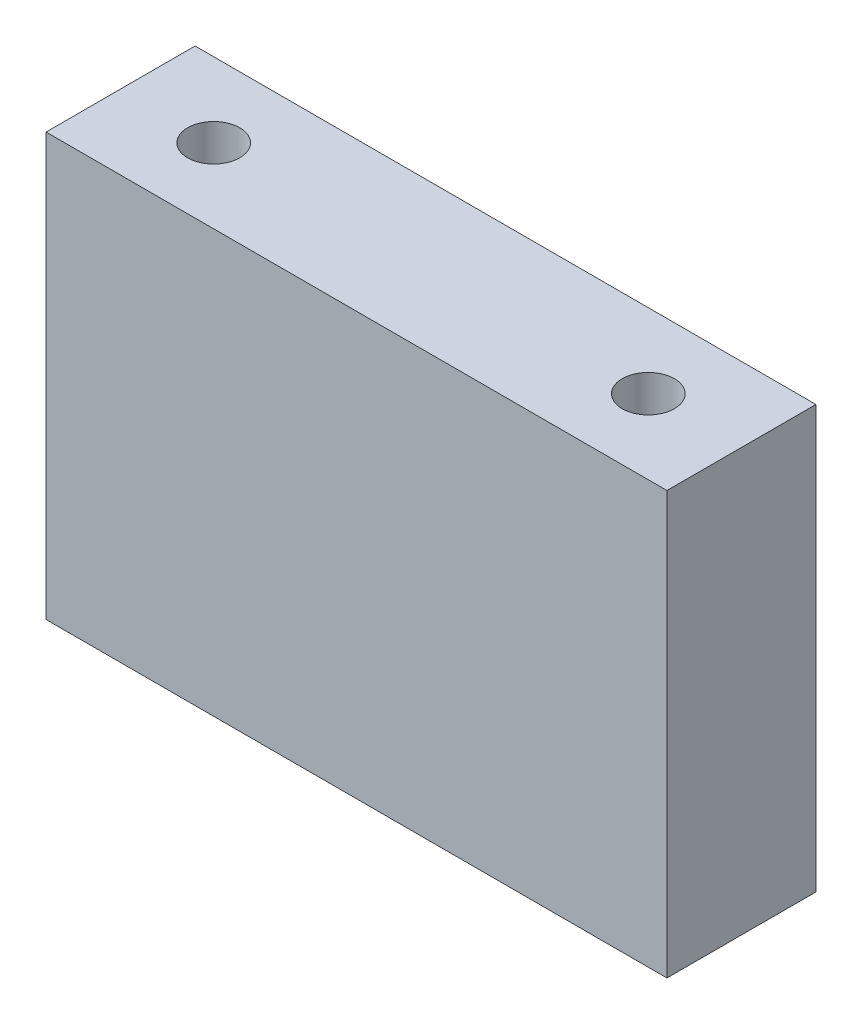
SolidWorks part; units mm, degrees
ref_plane "前视基准面" through (0, 0, 0) normal (0, 0, 1) x (1, 0, 0)
ref_plane "上视基准面" through (0, 0, 0) normal (0, 1, 0) x (1, 0, 0)
ref_plane "右视基准面" through (0, 0, 0) normal (1, 0, 0) x (0, 0, -1)
sketch "草图1" plane through (0, 0, 0) normal (0, 0, 1) x (1, 0, 0)
  line L1 (-25, -17) -> (25, -17)
  line L2 (-25, -17) -> (-25, 17)
  line L3 (-25, 17) -> (25, 17)
  line L4 (25, -17) -> (25, 17)
  line L5 (-25, -17) -> (25, 17) construction
  line L6 (-25, 17) -> (25, -17) construction
  point P0 (0, 0)
  dimension "D1" = 50
  dimension "D2" = 34
extrude "凸台-拉伸1" add sketch "草图1" along normal mid plane 12
sketch "草图4" plane through (0, -17, 0) normal (0, -1, 0) x (-1, 0, 0)
  point P0 (17.5, 0)
  point P3 (-17.5, 0)
hole_wizard "M5 螺纹孔1" positions "草图4" profile "草图3" tap size "M5" standard "GB"
sketch "草图3" plane through (-17.5, -17, 0) normal (1, 0, 0) x (0, 0, -1)
  line L0 (0, 0) -> (0, 13.6618)
  line L1 (0, 13.6618) -> (2.1, 12.4)
  line L2 (2.1, 12.4) -> (2.1, 0)
  line L5 (2.1, 0) -> (0, 0)
  line L10 (0, 13.6618) -> (-2.1, 12.4) construction
  line L11 (0, -6.35) -> (0, 107.95) construction
  dimension "螺纹孔钻头直径" = 4.2
  dimension "螺纹孔钻头深度" = 12.4
  dimension "导头角度" = 118
cosmetic thread "孔螺纹线1" parameters "D1"=10, "D2"=5
cosmetic thread "孔螺纹线2" parameters "D1"=10, "D2"=5
mirror "镜向1" about plane through (0, 0, 0) normal (0, 1, 0) of "M5 螺纹孔1"
